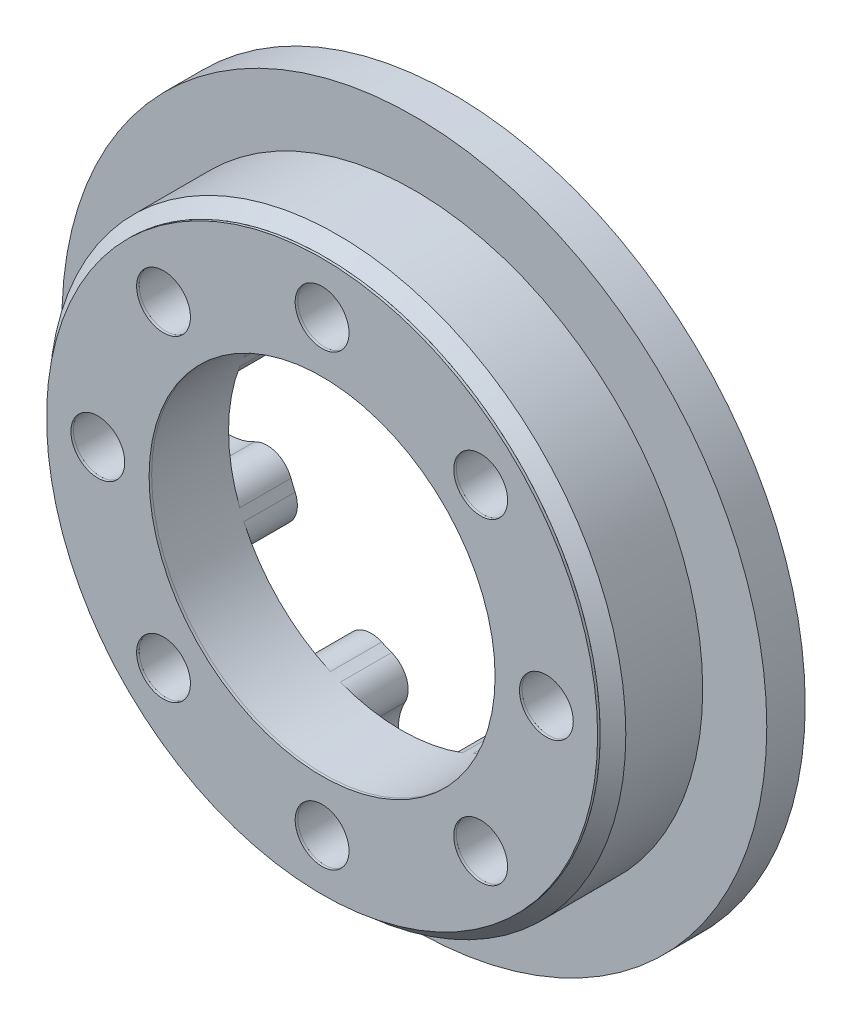
SolidWorks part; units mm, degrees
material "6061 合金"
ref_plane "前视基准面" through (0, 0, 0) normal (0, 0, 1) x (1, 0, 0)
ref_plane "上视基准面" through (0, 0, 0) normal (0, 1, 0) x (1, 0, 0)
ref_plane "右视基准面" through (0, 0, 0) normal (1, 0, 0) x (0, 0, -1)
other "Configuration Table"
sketch "草图1" plane through (0, 0, 0) normal (0, 1, 0) x (1, 0, 0)
  line L0 (0, -386.5023) -> (0, 18938.6108) construction
  line L1 (-27.5, 10) -> (-27.5, 7)
  line L2 (-27.5, 7) -> (-22.5, 7)
  line L3 (-22.5, 7) -> (-22.5, 0)
  line L4 (-22.5, 0) -> (-13.5, 0)
  line L5 (-13.5, 0) -> (-13.5, 10)
  line L6 (-13.5, 10) -> (-27.5, 10)
  dimension "D1" = 27
  dimension "D2" = 45
  dimension "D3" = 55
  dimension "D4" = 7
  dimension "D5" = 3
revolve "旋转1" add sketch "草图1" angle 360 about L0
sketch "草图2" plane through (0, 0, -10) normal (0, 0, -1) x (-1, 0, 0)
  circle A0 centre (0, 0) radius 17.5 construction
  circle A1 centre (0, 17.5) radius 2.1
  circle A2 centre (12.3744, 12.3744) radius 2.1
  circle A3 centre (17.5, 0) radius 2.1
  circle A4 centre (12.3744, -12.3744) radius 2.1
  circle A5 centre (0, -17.5) radius 2.1
  circle A6 centre (-12.3744, -12.3744) radius 2.1
  circle A7 centre (-17.5, 0) radius 2.1
  circle A8 centre (-12.3744, 12.3744) radius 2.1
  point P21 (0, 0)
  dimension "D1" = 35
  dimension "D2" = 4.2
  dimension "D3" = 8
extrude "切除-拉伸1" cut sketch "草图2" against normal through all
sketch "草图3" plane through (0, 0, -10) normal (0, 0, -1) x (-1, 0, 0)
  circle A0 centre (0, 0) radius 17.5 construction
  circle A1 centre (0, 17.5) radius 4.25
  circle A2 centre (12.3744, 12.3744) radius 4.25
  circle A3 centre (17.5, 0) radius 4.25
  circle A4 centre (12.3744, -12.3744) radius 4.25
  circle A5 centre (0, -17.5) radius 4.25
  circle A6 centre (-12.3744, -12.3744) radius 4.25
  circle A7 centre (-17.5, 0) radius 4.25
  circle A8 centre (-12.3744, 12.3744) radius 4.25
  dimension "D1" = 35
  dimension "D2" = 8.5
  dimension "D3" = 8
extrude "切除-拉伸5" cut sketch "草图3" against normal blind 4
fillet "圆角1" radius 2 16 edges at (13.4411, 1.26, -8) (13.4411, -1.26, -8) (10.3952, -8.6133, -8) (8.6133, -10.3952, -8) (1.26, -13.4411, -8) (-1.26, -13.4411, -8) (-8.6133, -10.3952, -8) (-10.3952, -8.6133, -8) (-13.4411, -1.26, -8) (-13.4411, 1.26, -8) (-10.3952, 8.6133, -8) (-8.6133, 10.3952, -8) (-1.26, 13.4411, -8) (1.26, 13.4411, -8) (8.6133, 10.3952, -8) (10.3952, 8.6133, -8)
chamfer "倒角2" distance 1 angle 45 1 edges at (22.5, 0, 0)
sketch "草图4" plane through (0, 0, 0) normal (0, 0, 1) x (1, 0, 0)
  circle A0 centre (0, 0) radius 21.5
  circle A1 centre (0, 0) radius 13.5
  circle A2 centre (0, 17.5) radius 2.1 construction
  circle A3 centre (-12.3744, 12.3744) radius 2.1 construction
  circle A4 centre (-17.5, 0) radius 2.1 construction
  circle A5 centre (-12.3744, -12.3744) radius 2.1 construction
  circle A6 centre (0, -17.5) radius 2.1 construction
  circle A7 centre (12.3744, -12.3744) radius 2.1 construction
  circle A8 centre (17.5, 0) radius 2.1 construction
  circle A9 centre (12.3744, 12.3744) radius 2.1 construction
  circle A10 centre (-12.3744, 12.3744) radius 2.1
  circle A11 centre (-17.5, 0) radius 2.1
  circle A12 centre (-12.3744, -12.3744) radius 2.1
  circle A13 centre (0, -17.5) radius 2.1
  circle A14 centre (12.3744, -12.3744) radius 2.1
  circle A15 centre (17.5, 0) radius 2.1
  circle A16 centre (12.3744, 12.3744) radius 2.1
  circle A17 centre (0, 17.5) radius 2.1
  dimension "D1" = 27
  dimension "D2" = 43
extrude "凸台-拉伸1" add sketch "草图4" along normal blind 0.2 separate body
